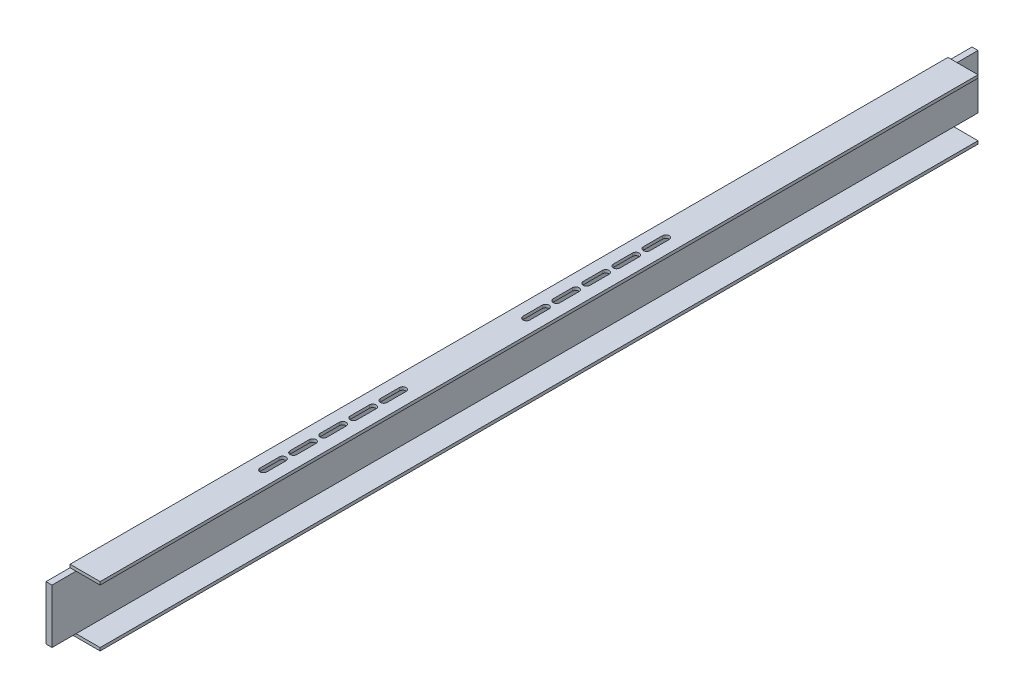
SolidWorks part; units mm, degrees
ref_plane "Front Plane" through (0, 0, 0) normal (0, 0, 1) x (1, 0, 0)
ref_plane "Top Plane" through (0, 0, 0) normal (0, 1, 0) x (1, 0, 0)
ref_plane "Right Plane" through (0, 0, 0) normal (1, 0, 0) x (0, 0, -1)
sketch "Sketch1" plane through (0, 0, 0) normal (0, 0, 1) x (1, 0, 0)
  line L0 (0, 0) -> (-40, 0)
  line L1 (-40, 0) -> (-40, 80)
  line L2 (-40, 80) -> (0, 80)
  line L3 (0, 80) -> (0, 76)
  line L4 (0, 76) -> (-32, 76)
  line L5 (-32, 76) -> (-32, 4)
  line L6 (-32, 4) -> (0, 4)
  line L7 (0, 4) -> (0, 0)
  dimension "D1" = 80
  dimension "D2" = 40
  dimension "D3" = 40
  dimension "D4" = 4
  dimension "D5" = 4
  dimension "D6" = 8
sheet metal parameters "Sheet metal 1" thickness 3 parameters "D1"=3
extrude "Extrude1" add sketch "Sketch1" along normal blind 1232
sketch "Sketch2" plane through (0, 80, 0) normal (0, 1, 0) x (1, 0, 0)
  line L0 (-40, -1232) -> (-40, 0) construction
  line L1 (0, 0) -> (-32, 0)
  line L2 (0, 0) -> (0, -32)
  line L3 (0, -32) -> (-32, -32)
  line L4 (-32, 0) -> (-32, -32)
  line L6 (0, -1232) -> (-32, -1232)
  line L7 (0, -1232) -> (0, -1200)
  line L8 (0, -1200) -> (-32, -1200)
  line L9 (-32, -1232) -> (-32, -1200)
  dimension "D1" = 8
  dimension "D2" = 32
  dimension "D3" = 8
  dimension "D4" = 32
extrude "Cut-Extrude1" cut sketch "Sketch2" against normal through all
sketch "Sketch3" plane through (-32, 0, 0) normal (1, 0, 0) x (0, 0, -1)
  line L1 (-1200, 76) -> (-1232, 76)
  line L2 (-1200, 76) -> (-1200, 80)
  line L3 (-1200, 80) -> (-1232, 80)
  line L4 (-1232, 76) -> (-1232, 80)
  line L5 (-1200, 4) -> (-1232, 4)
  line L6 (-1200, 4) -> (-1200, 0)
  line L7 (-1200, 0) -> (-1232, 0)
  line L8 (-1232, 4) -> (-1232, 0)
  line L9 (-32, 76) -> (0, 76)
  line L10 (-32, 76) -> (-32, 80)
  line L11 (-32, 80) -> (0, 80)
  line L12 (0, 76) -> (0, 80)
  line L14 (-32, 4) -> (0, 4)
  line L15 (-32, 4) -> (-32, 0)
  line L16 (-32, 0) -> (0, 0)
  line L17 (0, 4) -> (0, 0)
extrude "Cut-Extrude2" cut sketch "Sketch3" against normal blind 1200
sketch "Sketch4" plane through (0, 80, 0) normal (0, 1, 0) x (1, 0, 0)
  line L0 (-20, -937.25) -> (-20, -962.75) construction
  line L1 (0, -1200) -> (0, -32) construction
  line L2 (-24.5, -937.25) -> (-24.5, -962.75)
  line L3 (-15.5, -937.25) -> (-15.5, -962.75)
  arc A0 (-24.5, -937.25) -> (-15.5, -937.25) centre (-20, -937.25) cw
  arc A1 (-24.5, -962.75) -> (-15.5, -962.75) centre (-20, -962.75) ccw
  point P5 (-20, -950)
  dimension "D1" = 20
  dimension "D2" = 250
  dimension "D3" = 25.5
  dimension "D4" = 4.5
  dimension "D5" = 4.5
extrude "Cut-Extrude3" cut sketch "Sketch4" against normal blind 10
pattern_linear "LPattern1" count 5 spacing 40 along (0, 0, -1) of "Cut-Extrude3"
pattern_linear "LPattern2" count 2 spacing 350 along (0, 0, -1) of "Cut-Extrude3", "LPattern1"
